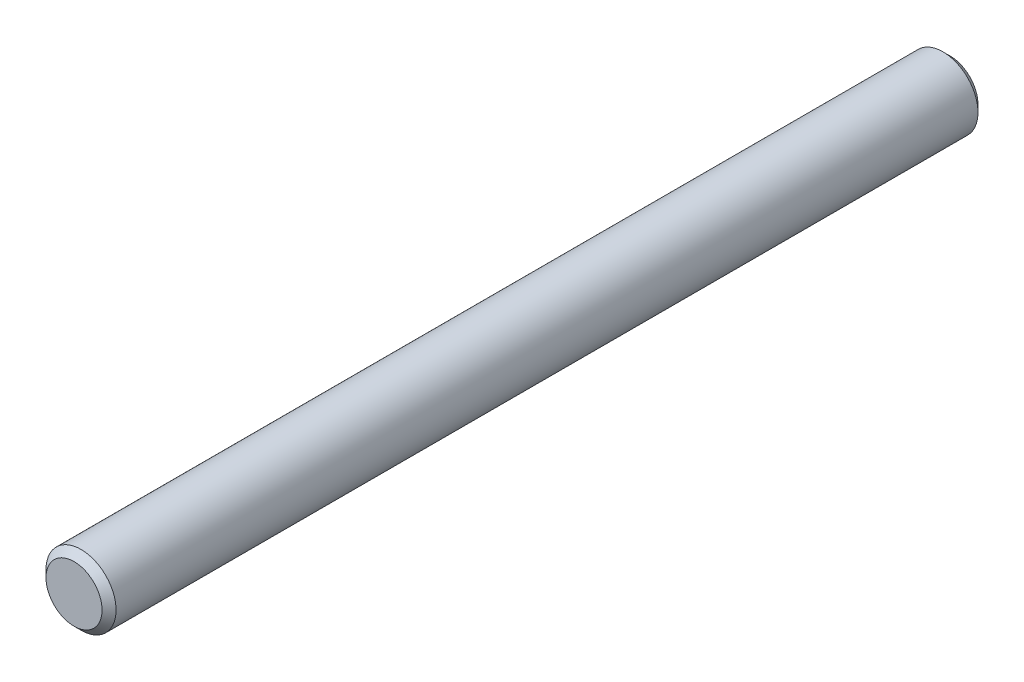
from build123d import *


with BuildPart() as part:
    # 草图1 → 旋转1 (revolve)
    with BuildSketch(Plane(origin=(0, 0, 0), x_dir=(1, 0, 0), z_dir=(0, 1, 0)), mode=Mode.PRIVATE) as revolve_1_sk:
        Polygon((0, 25), (0.8, 25), (1, 24.8), (1, 0.2), (0.8, 0), (0, 0), align=None)
    revolve(revolve_1_sk.sketch.rotate(Axis((0, 0, 0), (0, 0, -1)), 180), axis=Axis((0, 0, 0), (0, 0, -1)))


solid = part.part
